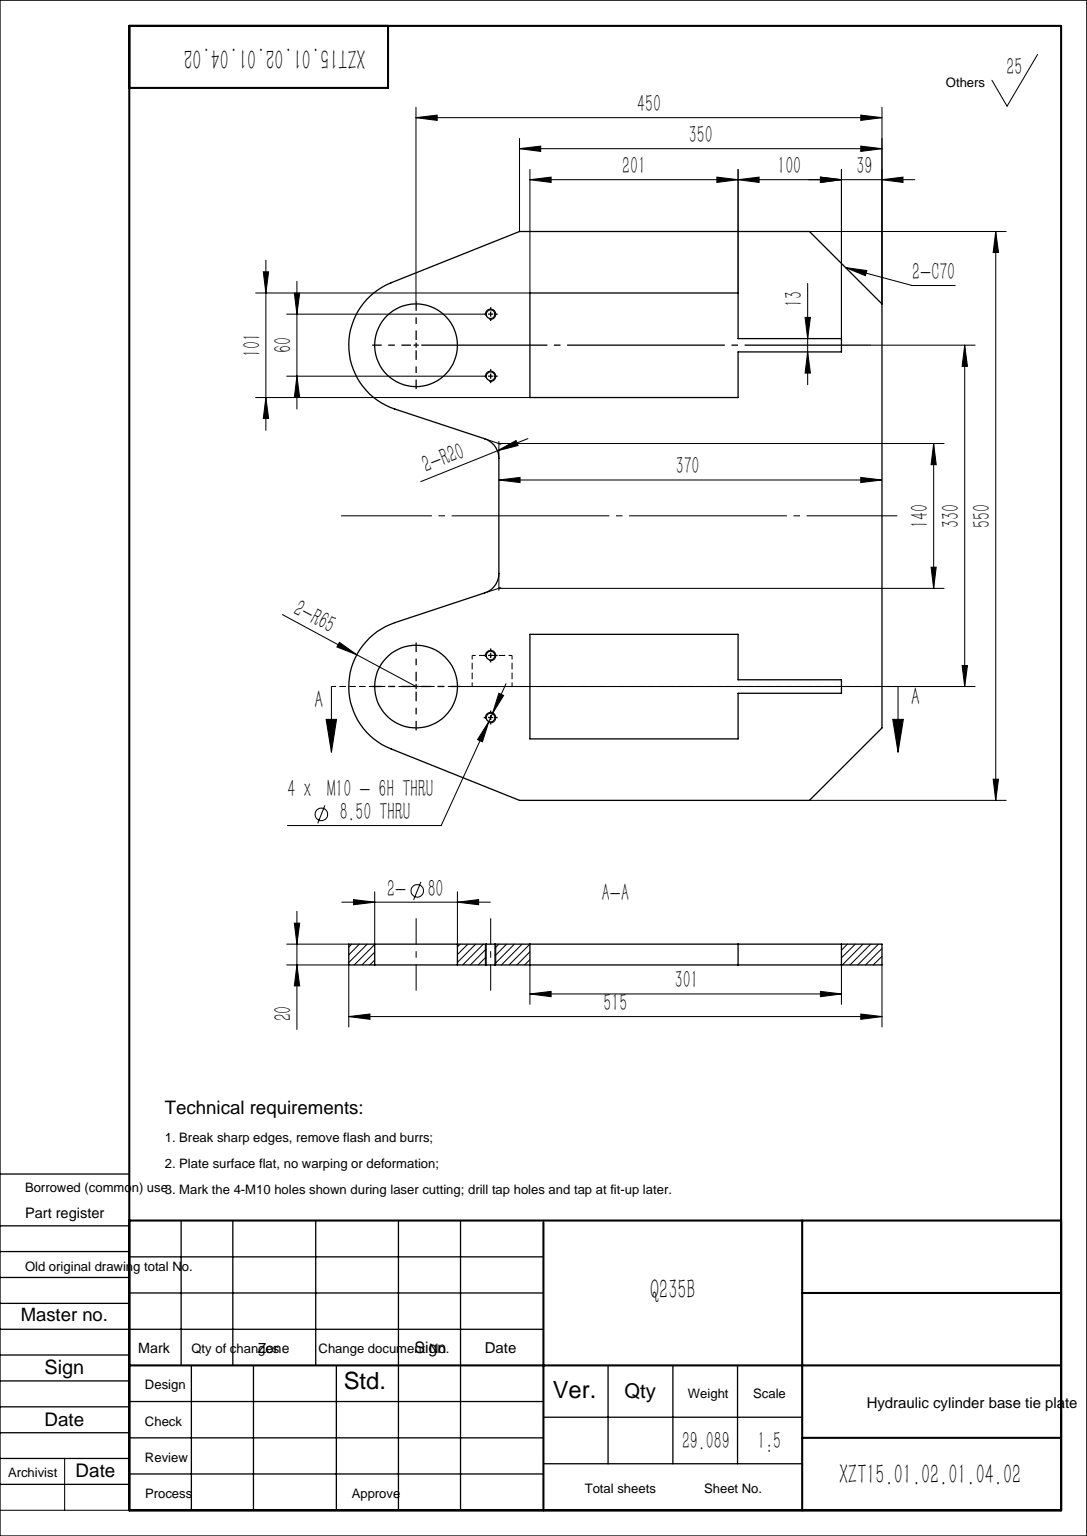
from build123d import *

# Parameters (mm, degrees)
SKETCH1_R           = 40
BOSS_EXTRUDE1_DEPTH = 20
M10_TAPPED_HOLE1_D  = 8.5
CHAMFER1_SIZE       = 70
FILLET1_R           = 20


with BuildPart() as part:
    # Sketch1 → Boss-Extrude1 (new body)
    with BuildSketch(Plane.XY):
        with BuildLine():
            Line((0, -70), (0, 70))
            Line((0, 70), (-100.453845954, 103.30202446))
            ThreePointArc((-100.453845954, 103.30202446), (-144.970416858, 163.039149842), (-104.13740045, 225.352182227))
            Line((-104.13740045, 225.352182227), (20, 275))
            Line((20, 275), (370, 275))
            Line((370, 275), (370, -275))
            Line((370, -275), (20, -275))
            Line((20, -275), (-104.13740045, -225.352182227))
            ThreePointArc((-104.13740045, -225.352182227), (-144.970416858, -163.039149842), (-100.453845954, -103.30202446))
            Line((-100.453845954, -103.30202446), (0, -70))
        make_face()
        with Locations((-80, 165)):
            Circle(SKETCH1_R, mode=Mode.SUBTRACT)
        with Locations(Location((-80, -165, 0), (0, 0, 180))):
            Circle(SKETCH1_R, mode=Mode.SUBTRACT)
        Polygon((231, 158.5), (231, 114.5), (30, 114.5), (30, 215.5), (231, 215.5), (231, 171.5), (331, 171.5), (331, 158.5), align=None, mode=Mode.SUBTRACT)
        Polygon((331, -171.5), (331, -158.5), (231, -158.5), (231, -114.5), (30, -114.5), (30, -215.5), (231, -215.5), (231, -171.5), align=None, mode=Mode.SUBTRACT)
    extrude(amount=BOSS_EXTRUDE1_DEPTH)

    # M10 Tapped Hole1 (through all)
    with Locations(Plane.XY.offset(20)):
        with Locations((-8, 195), (-8, 135), (-8, -135), (-8, -195)):
            Hole(M10_TAPPED_HOLE1_D / 2)

    # Chamfer1
    chamfer1_edges = [part.edges().sort_by_distance(p)[0] for p in [
        (370, 275, 10),
        (370, -275, 10),
    ]]
    chamfer(chamfer1_edges, length=CHAMFER1_SIZE)

    # Fillet1
    fillet1_edges = [part.edges().sort_by_distance(p)[0] for p in [
        (0, -70, 10),
        (0, 70, 10),
    ]]
    fillet(fillet1_edges, radius=FILLET1_R)


solid = part.part
